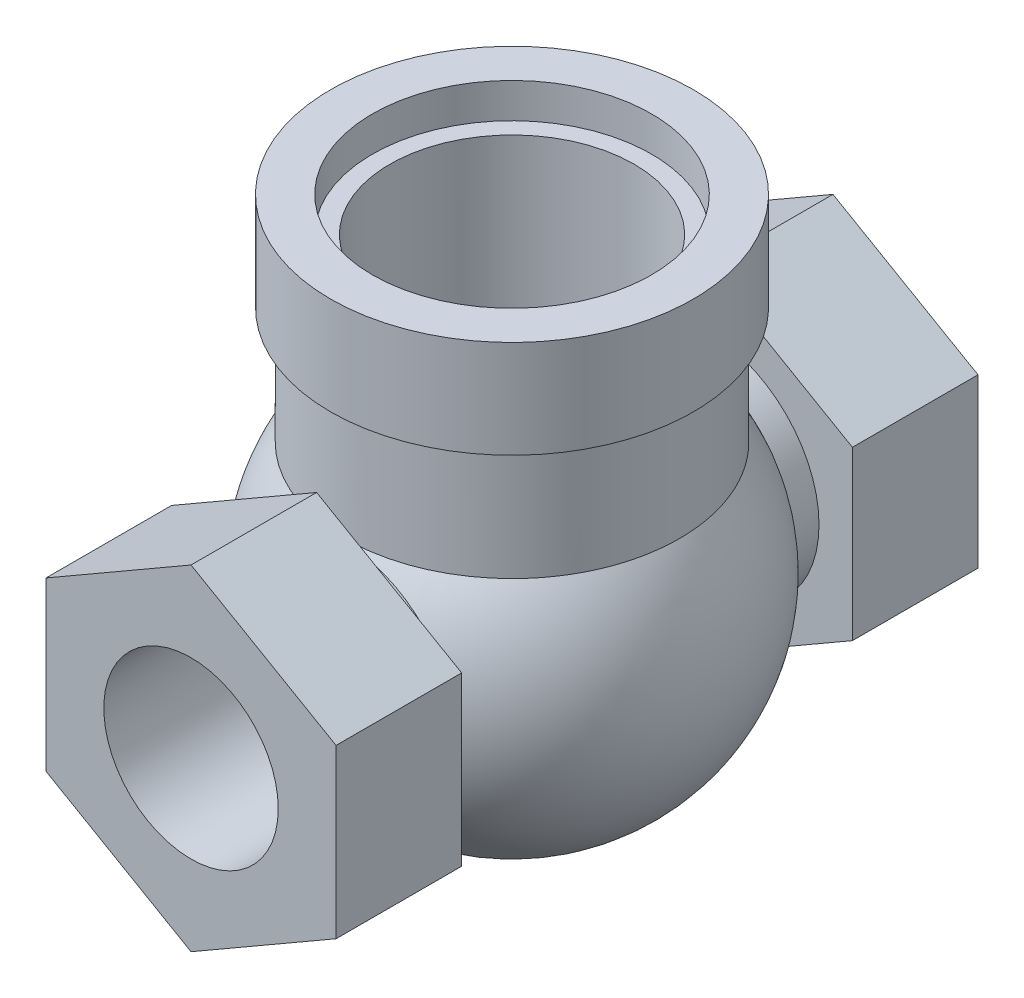
SolidWorks part; units mm, degrees
ref_plane "Front Plane" through (0, 0, 0) normal (0, 0, 1) x (1, 0, 0)
ref_plane "Top Plane" through (0, 0, 0) normal (0, 1, 0) x (1, 0, 0)
ref_plane "Right Plane" through (0, 0, 0) normal (1, 0, 0) x (0, 0, -1)
sketch "Sketch1" plane through (0, 0, 0) normal (0, 0, 1) x (1, 0, 0)
  line L0 (-1000, 0) -> (49000, 0) construction
  line L1 (-29, 0) -> (29, 0)
  arc A0 (29, 0) -> (-29, 0) centre (0, 0) ccw
  dimension "D1" = 58
revolve "Revolve1" add sketch "Sketch1" angle 360 about L0
sketch "Sketch2" plane through (0, 0, 0) normal (0, 1, 0) x (1, 0, 0)
  circle A0 centre (0, 0) radius 24
  dimension "D1" = 48
extrude "Boss-Extrude1" add sketch "Sketch2" along normal blind 47
sketch "Sketch3" plane through (0, 47, 0) normal (0, 1, 0) x (1, 0, 0)
  circle A0 centre (0, 0) radius 26
  dimension "D1" = 52
extrude "Boss-Extrude2" add sketch "Sketch3" against normal blind 14
sketch "Sketch4" plane through (0, 0, 0) normal (0, 0, 1) x (1, 0, 0)
  line L1 (20.7846, 12) -> (0, 24)
  line L2 (0, 24) -> (-20.7846, 12)
  line L3 (-20.7846, 12) -> (-20.7846, -12)
  line L4 (-20.7846, -12) -> (0, -24)
  line L5 (0, -24) -> (20.7846, -12)
  line L6 (20.7846, -12) -> (20.7846, 12)
  circle A0 centre (0, 0) radius 20.7846 construction
  dimension "D1" = 48
sketch "Sketch5" plane through (0, 0, 0) normal (0, 0, 1) x (1, 0, 0)
  circle A0 centre (0, 0) radius 16
  dimension "D1" = 32
extrude "Boss-Extrude3" add sketch "Sketch5" along normal blind 46
extrude "Boss-Extrude4" add sketch "Sketch4" along normal blind 18 from offset 28
sketch "Sketch8" plane through (0, 47, 0) normal (0, 1, 0) x (1, 0, 0)
  circle A0 centre (0, 0) radius 20
  dimension "D1" = 40
extrude "Cut-Extrude1" cut sketch "Sketch8" against normal blind 5
sketch "Sketch12" plane through (0, 0, 46) normal (0, 0, 1) x (1, 0, 0)
  circle A0 centre (0, 0) radius 12.5
  dimension "D1" = 25
extrude "Cut-Extrude3" cut sketch "Sketch12" against normal blind 34
mirror "Mirror1" about plane through (0, 0, 0) normal (0, 0, 1) of "Boss-Extrude4", "Boss-Extrude3"
sketch "Sketch13" plane through (0, 0, -46) normal (0, 0, -1) x (-1, 0, 0)
  circle A0 centre (0, 0) radius 12.5
  dimension "D1" = 25
extrude "Cut-Extrude4" cut sketch "Sketch13" against normal blind 25
sketch "Sketch11" plane through (0, 42, 0) normal (0, 1, 0) x (1, 0, 0)
  circle A0 centre (0, 0) radius 17.5
  dimension "D1" = 35
extrude "Cut-Extrude2" cut sketch "Sketch11" against normal blind 39
sketch "Sketch15" plane through (0, 0, 0) normal (1, 0, 0) x (0, 0, -1)
  line L0 (0, -1000) -> (0, 49000) construction
  line L1 (-6.5, 3) -> (0, -3.5)
  line L2 (17.5, 3) -> (-12.6095, 3) construction
  line L3 (-2.5, -1) -> (0, -1) construction
  line L6 (-6.5, 3) -> (-6.5, 11)
  line L7 (-6.5, 11) -> (0, 11)
  line L8 (0, -3.5) -> (0, 11)
  dimension "D1" = 45
  dimension "D2" = 4
  dimension "D3" = 2.5
  dimension "D4" = 8
revolve "Cut-Revolve1" cut sketch "Sketch15" angle 360 about L0
sketch "Sketch16" plane through (0, 0, 0) normal (1, 0, 0) x (0, 0, -1)
  line L0 (-4.897, -5) -> (49.0452, -5) construction
  line L1 (-2.5, -5) -> (-2.5, -7.5)
  line L2 (-2.5, -7.5) -> (26.5, -7.5)
  line L3 (26.5, -7.5) -> (26.5, -5)
  line L4 (-2.5, -5) -> (26.5, -5)
  dimension "D1" = 5
  dimension "D2" = 2.5
  dimension "D3" = 2.5
  dimension "D4" = 29
revolve "Cut-Revolve2" cut sketch "Sketch16" angle 360 about L0
sketch "Sketch17" plane through (0, 0, 0) normal (1, 0, 0) x (0, 0, -1)
  line L0 (-2.5, 6.4356) -> (-2.5, -5)
  line L2 (-2.5, -5) -> (0, -5)
  line L3 (0, -5) -> (0, 6.4356)
  line L4 (0, 6.4356) -> (-2.5, 6.4356)
  dimension "D1" = 2.5
  dimension "D2" = 11.4356
  dimension "D3" = 5
revolve "Cut-Revolve3" cut sketch "Sketch17" angle 360 about L3
